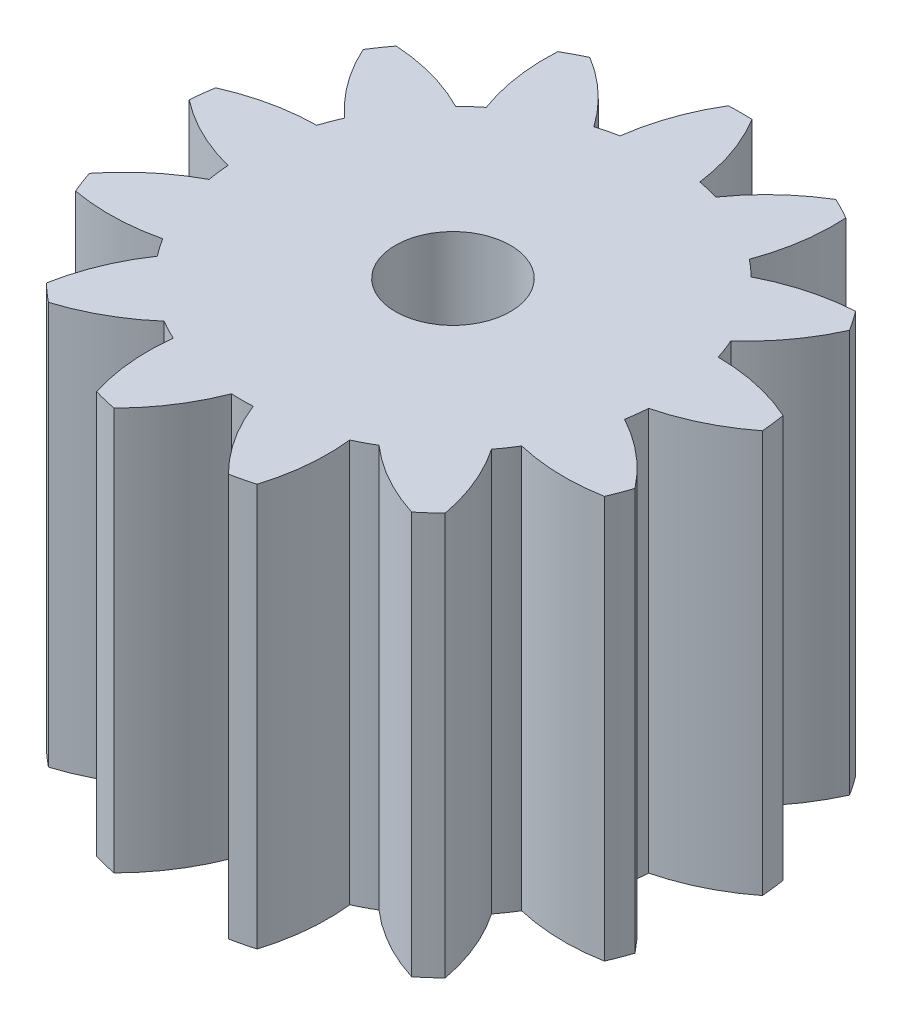
from build123d import *

# Parameters (mm, degrees)
BOSS_EXTRUDE1_DEPTH = 10.5
SKETCH2_R           = 1.5
CUT_EXTRUDE1_DEPTH  = 10.5


with BuildPart() as part:
    # Sketch1 → Boss-Extrude1 (new body)
    with BuildSketch(Plane(origin=(0, 0, 0), x_dir=(1, 0, 0), z_dir=(0, 1, 0))):
        with BuildLine():
            ThreePointArc((1.04, 5.400777722), (0.783531714, 6.485041414), (0.31, 7.493590595))
            ThreePointArc((0.31, 7.493590595), (0, 7.5), (-0.31, 7.493590595))
            ThreePointArc((-0.31, 7.493590595), (-0.783531714, 6.485041414), (-1.04, 5.400777722))
            ThreePointArc((-1.04, 5.400777722), (-1.316236154, 5.340179996), (-1.588992288, 5.265463276))
            ThreePointArc((-1.588992288, 5.265463276), (-2.319966139, 6.10634434), (-3.207953823, 6.779309129))
            ThreePointArc((-3.207953823, 6.779309129), (-3.48542379, 6.640920192), (-3.756936559, 6.491180762))
            ThreePointArc((-3.756936559, 6.491180762), (-3.707531894, 5.378093653), (-3.430740821, 4.298839078))
            ThreePointArc((-3.430740821, 4.298839078), (-3.64717462, 4.116809115), (-3.853965592, 3.923894649))
            ThreePointArc((-3.853965592, 3.923894649), (-4.891987708, 4.328757368), (-5.991004086, 4.511969642))
            ThreePointArc((-5.991004086, 4.511969642), (-6.172378994, 4.2604856), (-6.343204228, 4.001719645))
            ThreePointArc((-6.343204228, 4.001719645), (-5.782181198, 3.039089449), (-5.035540265, 2.212088208))
            ThreePointArc((-5.035540265, 2.212088208), (-5.142589335, 1.950326879), (-5.236041824, 1.683409046))
            ThreePointArc((-5.236041824, 1.683409046), (-6.343313848, 1.559504249), (-7.401587511, 1.210992284))
            ThreePointArc((-7.401587511, 1.210992284), (-7.445316556, 0.904025102), (-7.476320253, 0.595512782))
            ThreePointArc((-7.476320253, 0.595512782), (-6.532202472, 0.003866477), (-5.486758119, -0.381425412))
            ThreePointArc((-5.486758119, -0.381425412), (-5.459898808, -0.662951741), (-5.418603976, -0.942725282))
            ThreePointArc((-5.418603976, -0.942725282), (-6.341463231, -1.567012498), (-7.116556437, -2.367408811))
            ThreePointArc((-7.116556437, -2.367408811), (-7.01262182, -2.659536653), (-6.896701407, -2.947118882))
            ThreePointArc((-6.896701407, -2.947118882), (-5.785774881, -3.032242258), (-4.68102581, -2.887559066))
            ThreePointArc((-4.68102581, -2.887559066), (-4.526411262, -3.124356107), (-4.359829258, -3.352892609))
            ThreePointArc((-4.359829258, -3.352892609), (-4.886859811, -4.334545567), (-5.201208047, -5.403465078))
            ThreePointArc((-5.201208047, -5.403465078), (-4.973419937, -5.613830611), (-4.737131383, -5.814601127))
            ThreePointArc((-4.737131383, -5.814601127), (-3.713895991, -5.373700834), (-2.802926901, -4.732187738))
            ThreePointArc((-2.802926901, -4.732187738), (-2.555977446, -4.870008141), (-2.302270198, -4.994952646))
            ThreePointArc((-2.302270198, -4.994952646), (-2.312735701, -6.109086484), (-2.094325574, -7.201652615))
            ThreePointArc((-2.094325574, -7.201652615), (-1.794867482, -7.282063631), (-1.492341648, -7.350028327))
            ThreePointArc((-1.492341648, -7.350028327), (-0.791208287, -6.484109309), (-0.282711218, -5.492729228))
            ThreePointArc((-0.282711218, -5.492729228), (0, -5.5), (0.282711218, -5.492729228))
            ThreePointArc((0.282711218, -5.492729228), (0.791208287, -6.484109309), (1.492341648, -7.350028327))
            ThreePointArc((1.492341648, -7.350028327), (1.794867482, -7.282063631), (2.094325574, -7.201652615))
            ThreePointArc((2.094325574, -7.201652615), (2.312735701, -6.109086484), (2.302270198, -4.994952646))
            ThreePointArc((2.302270198, -4.994952646), (2.555977446, -4.870008141), (2.802926901, -4.732187738))
            ThreePointArc((2.802926901, -4.732187738), (3.713895991, -5.373700834), (4.737131383, -5.814601127))
            ThreePointArc((4.737131383, -5.814601127), (4.973419937, -5.613830611), (5.201208047, -5.403465078))
            ThreePointArc((5.201208047, -5.403465078), (4.886859811, -4.334545567), (4.359829258, -3.352892609))
            ThreePointArc((4.359829258, -3.352892609), (4.526411262, -3.124356107), (4.68102581, -2.887559066))
            ThreePointArc((4.68102581, -2.887559066), (5.785774881, -3.032242258), (6.896701407, -2.947118882))
            ThreePointArc((6.896701407, -2.947118882), (7.01262182, -2.659536653), (7.116556437, -2.367408811))
            ThreePointArc((7.116556437, -2.367408811), (6.341463231, -1.567012498), (5.418603976, -0.942725282))
            ThreePointArc((5.418603976, -0.942725282), (5.459898808, -0.662951741), (5.486758119, -0.381425412))
            ThreePointArc((5.486758119, -0.381425412), (6.532202472, 0.003866477), (7.476320253, 0.595512782))
            ThreePointArc((7.476320253, 0.595512782), (7.445316556, 0.904025102), (7.401587511, 1.210992284))
            ThreePointArc((7.401587511, 1.210992284), (6.343313848, 1.559504249), (5.236041824, 1.683409046))
            ThreePointArc((5.236041824, 1.683409046), (5.142589335, 1.950326879), (5.035540265, 2.212088208))
            ThreePointArc((5.035540265, 2.212088208), (5.782181198, 3.039089449), (6.343204228, 4.001719645))
            ThreePointArc((6.343204228, 4.001719645), (6.172378994, 4.2604856), (5.991004086, 4.511969642))
            ThreePointArc((5.991004086, 4.511969642), (4.891987708, 4.328757368), (3.853965592, 3.923894649))
            ThreePointArc((3.853965592, 3.923894649), (3.64717462, 4.116809115), (3.430740821, 4.298839078))
            ThreePointArc((3.430740821, 4.298839078), (3.707531894, 5.378093653), (3.756936559, 6.491180762))
            ThreePointArc((3.756936559, 6.491180762), (3.48542379, 6.640920192), (3.207953823, 6.779309129))
            ThreePointArc((3.207953823, 6.779309129), (2.319966139, 6.10634434), (1.588992288, 5.265463276))
            ThreePointArc((1.588992288, 5.265463276), (1.316236154, 5.340179996), (1.04, 5.400777722))
        make_face()
    extrude(amount=BOSS_EXTRUDE1_DEPTH)

    # Sketch2 → Cut-Extrude1 (cut)
    with BuildSketch(Plane(origin=(0, 10.5, 0), x_dir=(1, 0, 0), z_dir=(0, 1, 0))):
        with Locations(Location((0, 0, 0), (0, 0, 270))):
            Circle(SKETCH2_R)
    extrude(amount=-CUT_EXTRUDE1_DEPTH, mode=Mode.SUBTRACT)


solid = part.part
